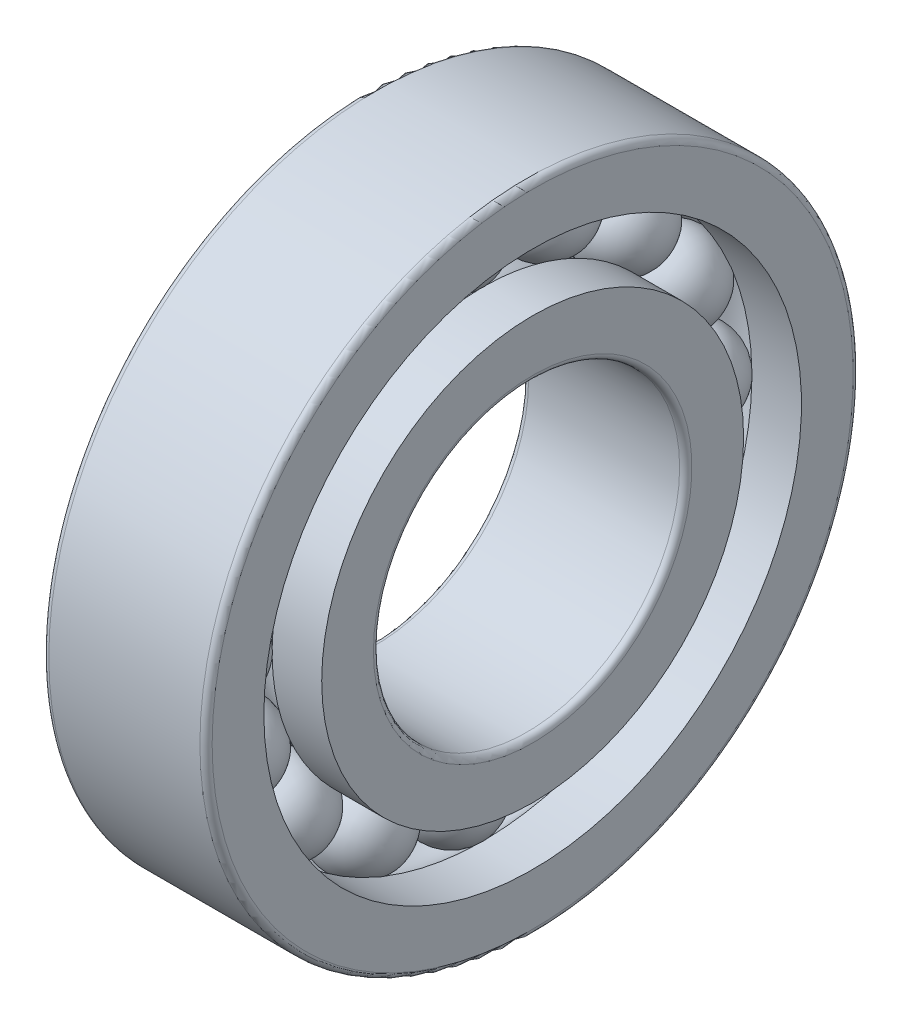
from build123d import *

# Parameters (mm, degrees)
CIRCULAR_PATTERN1_COUNT = 16
FILLET1_R               = 0.3


with BuildPart() as part:
    # Sketch1 → Revolve1 (revolve)
    with BuildSketch(Plane.XY):
        with BuildLine():
            Line((-2.125, 11.75), (2.125, 11.75))
            ThreePointArc((2.125, 11.75), (1.3e-16, 13.875), (-2.125, 11.75))
        make_face()
    revolve1 = revolve(axis=Axis((-4.596601835273904, 11.75, 0), (1, 0, 0)))

    # Sketch2 → Revolve2 (revolve)
    with BuildSketch(Plane.XY, mode=Mode.PRIVATE) as revolve2_sk:
        with BuildLine():
            Line((-4.000000000000001, 10.333333333333334), (-4, 7.5))
            Line((-4, 7.5), (4, 7.5))
            Line((4, 7.5), (4, 10.333333333333334))
            Line((4, 10.333333333333334), (1.5704396058287484, 10.333333333333334))
            ThreePointArc((1.5704396058287484, 10.333333333333334), (1.3e-16, 9.635000000000002), (-1.5704396058287484, 10.333333333333334))
            Line((-1.5704396058287484, 10.333333333333334), (-4.000000000000001, 10.333333333333334))
        make_face()
    revolve(revolve2_sk.sketch.rotate(Axis((-6.971390126215839, 0, 0), (1, 0, 0)), 90), axis=Axis((-6.971390126215839, 0, 0), (1, 0, 0)))

    # Sketch3 → Revolve3 (revolve)
    with BuildSketch(Plane.XY, mode=Mode.PRIVATE) as revolve3_sk:
        with BuildLine():
            Line((-4.000000000000002, 16), (3.9999999999999982, 16))
            Line((3.9999999999999982, 16), (3.9999999999999982, 13.166666666666666))
            Line((3.9999999999999982, 13.166666666666666), (1.5704396058287489, 13.166666666666666))
            ThreePointArc((1.5704396058287489, 13.166666666666666), (1.3e-16, 13.865), (-1.5704396058287489, 13.166666666666666))
            Line((-1.5704396058287489, 13.166666666666666), (-4.000000000000002, 13.166666666666666))
            Line((-4.000000000000002, 13.166666666666666), (-4.000000000000002, 16))
        make_face()
    revolve(revolve3_sk.sketch.rotate(Axis((-8.710676494715049, 0, 0), (1, 0, 0)), 90), axis=Axis((-8.710676494715049, 0, 0), (1, 0, 0)))

    # Circular-Pattern1: Revolve1 ×16 about axis
    circular_pattern1_axis = Axis((0, -1.3e-16, 2.1e-16), (1, 0, 0))
    for i in range(1, CIRCULAR_PATTERN1_COUNT):
        add(revolve1.rotate(circular_pattern1_axis, i * 360 / CIRCULAR_PATTERN1_COUNT))

    # Fillet1
    fillet1_edges = [part.edges().sort_by_distance(p)[0] for p in [
        (-4.000000000000002, -3.74e-15, -16),
        (3.9999999999999982, -3.74e-15, -16),
        (-4, -5.08e-15, -7.5),
        (4, -5.08e-15, -7.5),
    ]]
    fillet(fillet1_edges, radius=FILLET1_R)


solid = part.part
